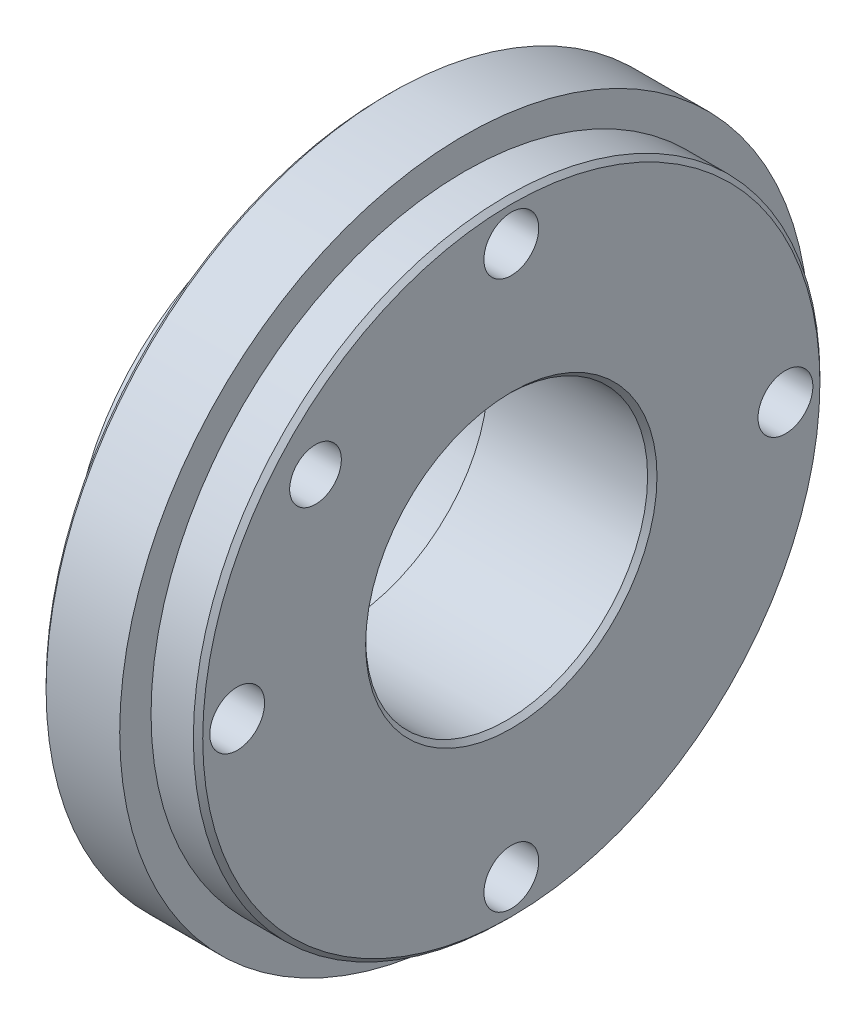
from build123d import *

# Parameters (mm, degrees)
CUT_EXTRUDE1_DEPTH  = 15
SKETCH4_R           = 10.25
CUT_EXTRUDE2_DEPTH  = 3.5
SKETCH5_R           = 1.75
CUT_EXTRUDE3_DEPTH  = 5
SKETCH7_R           = 20
SKETCH7_R_2         = 1.75
SKETCH7_R_3         = 9
BOSS_EXTRUDE1_DEPTH = 3
CUT_EXTRUDE5_REACH  = 36.321
SKETCH10_R          = 1.65
CHAMFER1_SIZE       = 0.3
CHAMFER2_SIZE       = 0.3


with BuildPart() as part:
    # Sketch1 → Revolve1 (revolve)
    with BuildSketch(Plane.XY, mode=Mode.PRIVATE) as revolve1_sk:
        Polygon((0, 9), (0, 14), (15, 14), (15, 22), (20, 22), (20, 9), align=None)
    revolve(revolve1_sk.sketch.rotate(Axis((0, 0, 0), (1, 0, 0)), 90), axis=Axis((0, 0, 0), (1, 0, 0)))

    # Sketch3 → Cut-Extrude1 (cut, symmetric)
    with BuildSketch(Plane.XY):
        Polygon((9.613311632, 17.562947239), (8.386688368, -17.562947239), (-5.415654366, -17.562947239), (-5.415654366, 17.562947239), align=None)
    extrude(amount=CUT_EXTRUDE1_DEPTH, both=True, mode=Mode.SUBTRACT)

    # Sketch4 → Cut-Extrude2 (cut)
    with BuildSketch(Plane(origin=(8.989038226, -0.313904132, 0), x_dir=(0, 0, 1), z_dir=(-0.9993908270190958, 0.03489949670250087, 0))):
        with Locations(Location((0, 0, 0), (0, 0, 270))):
            Circle(SKETCH4_R)
    extrude(amount=-CUT_EXTRUDE2_DEPTH, mode=Mode.SUBTRACT)

    # Sketch5 → Cut-Extrude3 (cut)
    with BuildSketch(Plane.ZY.offset(-15)):
        with Locations((-17.5, 0)):
            Circle(SKETCH5_R)
        with Locations((0, 17.5)):
            Circle(SKETCH5_R)
        with Locations((17.5, 0)):
            Circle(SKETCH5_R)
        with Locations((0, -17.5)):
            Circle(SKETCH5_R)
    extrude(amount=-CUT_EXTRUDE3_DEPTH, mode=Mode.SUBTRACT)

    # Sketch7 → Boss-Extrude1 (add)
    with BuildSketch(Plane(origin=(20, 0, 0), x_dir=(0, 0, -1), z_dir=(1, 0, 0))):
        with Locations(Location((0, 0, 0), (0, 0, 180))):
            Circle(SKETCH7_R)
        with Locations(Location((17.5, 0, 0), (0, 0, 180))):
            Circle(SKETCH7_R_2, mode=Mode.SUBTRACT)
        with Locations(Location((0, -17.5, 0), (0, 0, 180))):
            Circle(SKETCH7_R_2, mode=Mode.SUBTRACT)
        with Locations(Location((-17.5, 0, 0), (0, 0, 180))):
            Circle(SKETCH7_R_2, mode=Mode.SUBTRACT)
        with Locations(Location((0, 17.5, 0), (0, 0, 180))):
            Circle(SKETCH7_R_2, mode=Mode.SUBTRACT)
        with Locations(Location((0, 0, 0), (0, 0, 270))):
            Circle(SKETCH7_R_3, mode=Mode.SUBTRACT)
    extrude(amount=BOSS_EXTRUDE1_DEPTH)

    # Sketch10 → Cut-Extrude5 (cut, up to next)
    with BuildSketch(Plane(origin=(23, 0, 0), x_dir=(0, 0, -1), z_dir=(1, 0, 0)), mode=Mode.PRIVATE) as cut_extrude5_sk1:
        with Locations((-12.5, 11)):
            Circle(SKETCH10_R)
    cut_extrude5_tool1 = extrude(cut_extrude5_sk1.sketch, amount=-CUT_EXTRUDE5_REACH, mode=Mode.PRIVATE) & part.part
    add(cut_extrude5_tool1.solids().sort_by_distance((23, 11, 12.5))[0], mode=Mode.SUBTRACT)

    # Chamfer1
    chamfer1_edges = [part.edges().sort_by_distance(p)[0] for p in [
        (23, 0, -20),
        (15, 0, -22),
    ]]
    chamfer(chamfer1_edges, length=CHAMFER1_SIZE)

    # Chamfer2
    chamfer2_edges = [part.edges().sort_by_distance(p)[0] for p in [
        (23, 9, 0),
    ]]
    chamfer(chamfer2_edges, length=CHAMFER2_SIZE)


solid = part.part
